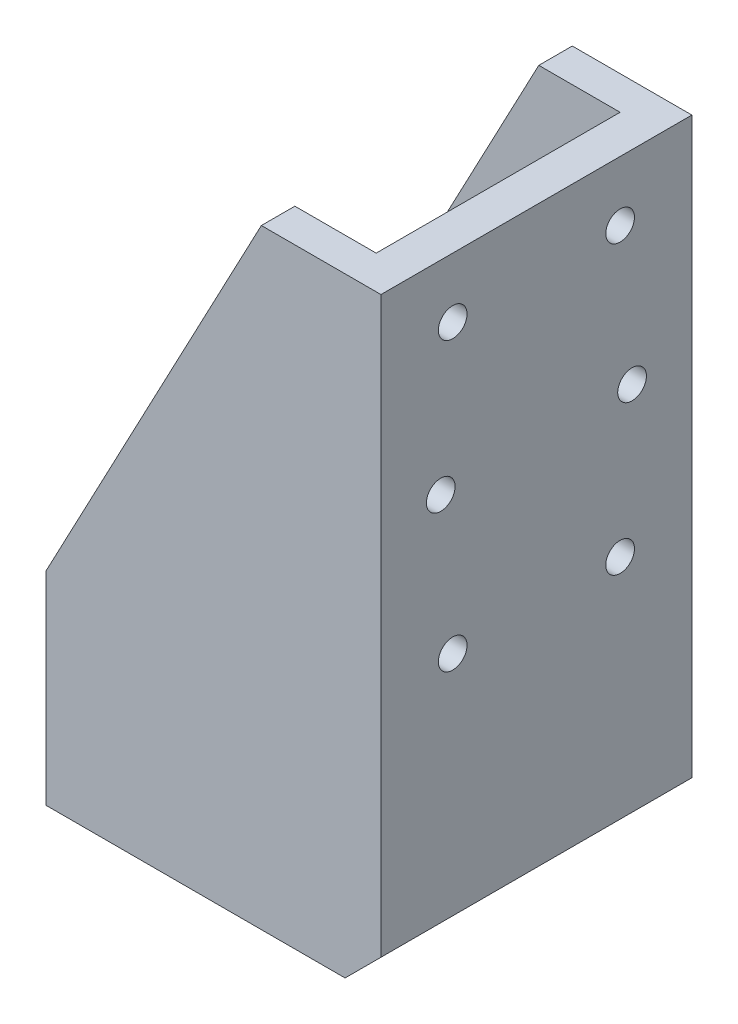
SolidWorks part; units mm, degrees
ref_plane "前视基准面" through (0, 0, 0) normal (0, 0, 1) x (1, 0, 0)
ref_plane "上视基准面" through (0, 0, 0) normal (0, 1, 0) x (1, 0, 0)
ref_plane "右视基准面" through (0, 0, 0) normal (1, 0, 0) x (0, 0, -1)
other "Configuration Table"
sketch "草图1" plane through (0, 0, 0) normal (0, 0, 1) x (1, 0, 0)
  line L0 (0, 0) -> (-140, 0)
  line L1 (-140, 0) -> (-140, 90)
  line L2 (-140, 90) -> (-50, 260)
  line L3 (-50, 260) -> (0, 260)
  line L4 (0, 260) -> (0, 0)
  dimension "D1" = 260
  dimension "D2" = 140
  dimension "D3" = 90
  dimension "D4" = 50
extrude "凸台-拉伸1" add sketch "草图1" along normal blind 130
sketch "草图2" plane through (0, 0, 130) normal (0, 0, 1) x (1, 0, 0)
  line L4 (-140, 90) -> (-140, 0) construction
  line L5 (0, 0) -> (-140, 0)
  line L6 (0, 0) -> (0, 5)
  line L7 (0, 5) -> (-140, 5)
  line L8 (-140, 0) -> (-140, 5)
  dimension "D1" = 5
extrude "切除-拉伸1" cut sketch "草图2" against normal through all
sketch "草图3" plane through (-140, 34.7726, 0) normal (1, 0, 0) x (0, 0, -1)
  line L1 (-116, 225.2274) -> (-14, 225.2274)
  line L2 (-116, 225.2274) -> (-116, 55.2274)
  line L3 (-116, 55.2274) -> (-14, 55.2274)
  line L4 (-14, 225.2274) -> (-14, 55.2274)
  line L5 (-130, -29.7726) -> (-130, 225.2274) construction
  line L6 (0, -29.7726) -> (0, 225.2274) construction
  line L7 (-130, 225.2274) -> (0, 225.2274) construction
  line L8 (-130, 55.2274) -> (0, 55.2274) construction
  dimension "D1" = 14
  dimension "D2" = 14
  dimension "D3" = 0
extrude "切除-拉伸2" cut sketch "草图3" along normal offset from surface (124 mm away) 16 up to face at (0, 132.5, 65)
sketch "草图5" plane through (0, 0, 130) normal (0, 0, 1) x (1, 0, 0)
  line L7 (0, 5) -> (0, 20)
  line L8 (0, 5) -> (0, 260) construction
  line L9 (0, 20) -> (-15, 5)
  line L10 (0, 5) -> (-140, 5) construction
  line L11 (-15, 5) -> (0, 5)
  dimension "D1" = 15
  dimension "D2" = 45
extrude "切除-拉伸3" cut sketch "草图5" against normal through all
sketch "草图8" plane through (0, 0, 0) normal (1, 0, 0) x (0, 0, -1)
  line L0 (-130, 260) -> (0, 260) construction
  line L1 (-130, 20) -> (-130, 260) construction
  line L2 (0, 20) -> (0, 260) construction
  line L3 (-30, 235) -> (-30, 115) construction
  point P0 (-100, 235)
  point P7 (-30, 235)
  point P18 (-100, 115)
  point P19 (-30, 115)
  dimension "D1" = 25
  dimension "D2" = 30
  dimension "D3" = 30
  dimension "D4" = 25
  dimension "D6" = 120
  dimension "D5" = 2
hole_wizard "M14 螺纹孔1" positions "草图8" profile "草图7" tap size "M14" standard "GB"
sketch "草图7" plane through (0, 235, 100) normal (0, 1, 0) x (0, 0, -1)
  line L0 (0, 0) -> (0, 37.6052)
  line L1 (0, 37.6052) -> (6, 34)
  line L2 (6, 34) -> (6, 0)
  line L5 (6, 0) -> (0, 0)
  line L10 (0, 37.6052) -> (-6, 34) construction
  line L11 (0, -6.35) -> (0, 107.95) construction
  dimension "螺纹孔钻头直径" = 12
  dimension "螺纹孔钻头深度" = 34
  dimension "导头角度" = 118
cosmetic thread "孔螺纹线1" parameters "D1"=28, "D2"=14
cosmetic thread "孔螺纹线2" parameters "D1"=28, "D2"=14
cosmetic thread "孔螺纹线3" parameters "D1"=28, "D2"=14
cosmetic thread "孔螺纹线4" parameters "D1"=28, "D2"=14
sketch "草图11" plane through (0, 0, 0) normal (1, 0, 0) x (0, 0, -1)
  line L0 (-130, 20) -> (-130, 260) construction
  line L1 (-130, 260) -> (0, 260) construction
  line L2 (0, 20) -> (0, 260) construction
  point P0 (-105, 175)
  point P2 (-25, 175)
  dimension "D1" = 25
  dimension "D2" = 85
  dimension "D3" = 25
  dimension "D4" = 85
hole_wizard "Ø12.0 (12) 直径孔1" positions "草图11" profile "草图10" hole size "Ø12.0" standard "GB"
sketch "草图10" plane through (0, 175, 105) normal (0, 1, 0) x (0, 0, -1)
  line L0 (0, 0) -> (0, 37.6052)
  line L1 (0, 37.6052) -> (6, 34)
  line L2 (6, 34) -> (6, 0)
  line L5 (6, 0) -> (0, 0)
  line L10 (0, 37.6052) -> (-6, 34) construction
  line L11 (0, -6.35) -> (0, 107.95) construction
  dimension "孔直径" = 12
  dimension "孔深度" = 34
  dimension "导头角度" = 118
sketch "草图12" plane through (-90.854, 5, 0) normal (0, 1, 0) x (-1, 0, 0)
  line L0 (49.146, 116) -> (49.146, 14) construction
  line L2 (-75.854, 0) -> (49.146, 0) construction
  circle A0 centre (-0.854, 63) radius 22.5
  dimension "D3" = 45
  dimension "D2" = 63
  dimension "D1" = 50
extrude "切除-拉伸4" cut sketch "草图12" along normal up to next
